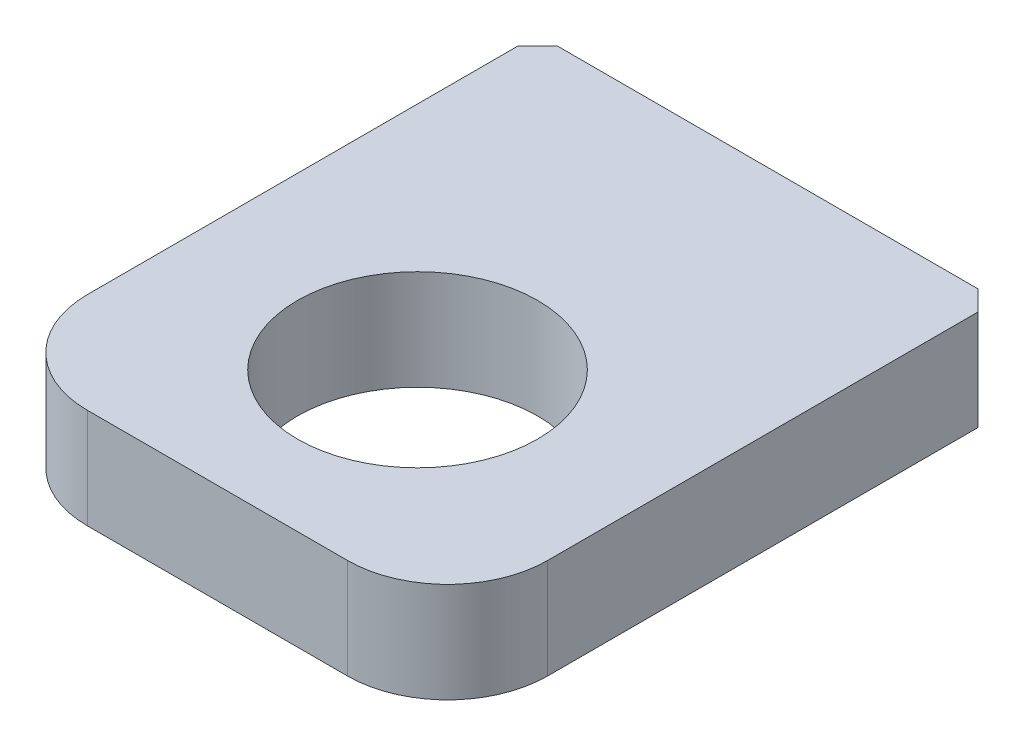
SolidWorks part; units mm, degrees
material "6061 合金"
ref_plane "前视基准面" through (0, 0, 0) normal (0, 0, 1) x (1, 0, 0)
ref_plane "上视基准面" through (0, 0, 0) normal (0, 1, 0) x (1, 0, 0)
ref_plane "右视基准面" through (0, 0, 0) normal (1, 0, 0) x (0, 0, -1)
sketch "草图1" plane through (0, 0, 0) normal (0, 1, 0) x (1, 0, 0)
  line L1 (-23, 27.5) -> (23, 27.5)
  line L2 (-23, 27.5) -> (-23, -27.5)
  line L3 (-23, -27.5) -> (23, -27.5)
  line L4 (23, 27.5) -> (23, -27.5)
  line L5 (-23, 27.5) -> (23, -27.5) construction
  line L6 (-23, -27.5) -> (23, 27.5) construction
  point P0 (0, 0)
  dimension "D1" = 46
  dimension "D2" = 55
extrude "凸台-拉伸1" add sketch "草图1" along normal mid plane 10
hole_wizard "M27*1.0反牙" positions "草图3" profile "草图2" tap size "M27" standard "GB" end condition up to next
sketch "草图3" plane through (0, 5, 0) normal (0, 1, 0) x (1, 0, 0)
  line L1 (-23, -27.5) -> (23, -27.5) construction
  point P0 (0, -7.5)
  dimension "D1" = 20
sketch "草图2" plane through (0, 5, 7.5) normal (1, 0, 0) x (0, 0, 1)
  line L0 (0, 0) -> (0, 10)
  line L1 (0, 10) -> (12, 10)
  line L2 (12, 10) -> (12, 0)
  line L5 (12, 0) -> (0, 0)
  line L11 (0, -6.35) -> (0, 107.95) construction
  dimension "通孔螺纹孔钻头直径" = 24
  dimension "通孔螺纹孔钻头深度" = 10
cosmetic thread "孔螺蚊线1" parameters "D2"=27
fillet "圆角1" radius 10 2 edges at (23, 0, 27.5) (-23, 0, 27.5)
hole_wizard "M4 螺纹孔1" positions "草图5" profile "草图4" tap size "M4" standard "GB"
sketch "草图5" plane through (0, 0, -27.5) normal (0, 0, -1) x (-1, 0, 0)
  point P0 (-15, 0)
  point P2 (15, 0)
  dimension "D1" = 15
  dimension "D2" = 15
sketch "草图4" plane through (15, 0, -27.5) normal (1, 0, 0) x (0, 1, 0)
  line L0 (0, 0) -> (0, 12.4914)
  line L1 (0, 12.4914) -> (1.65, 11.5)
  line L2 (1.65, 11.5) -> (1.65, 0)
  line L5 (1.65, 0) -> (0, 0)
  line L10 (0, 12.4914) -> (-1.65, 11.5) construction
  line L11 (0, -6.35) -> (0, 107.95) construction
  dimension "螺纹孔钻头直径" = 3.3
  dimension "螺纹孔钻头深度" = 11.5
  dimension "导头角度" = 118
cosmetic thread "孔螺蚊线2" parameters "D1"=8, "D2"=4
cosmetic thread "孔螺蚊线3" parameters "D1"=8, "D2"=4
chamfer "倒角1" distance 2 angle 45 2 edges at (23, 0, -27.5) (-23, 0, -27.5)
